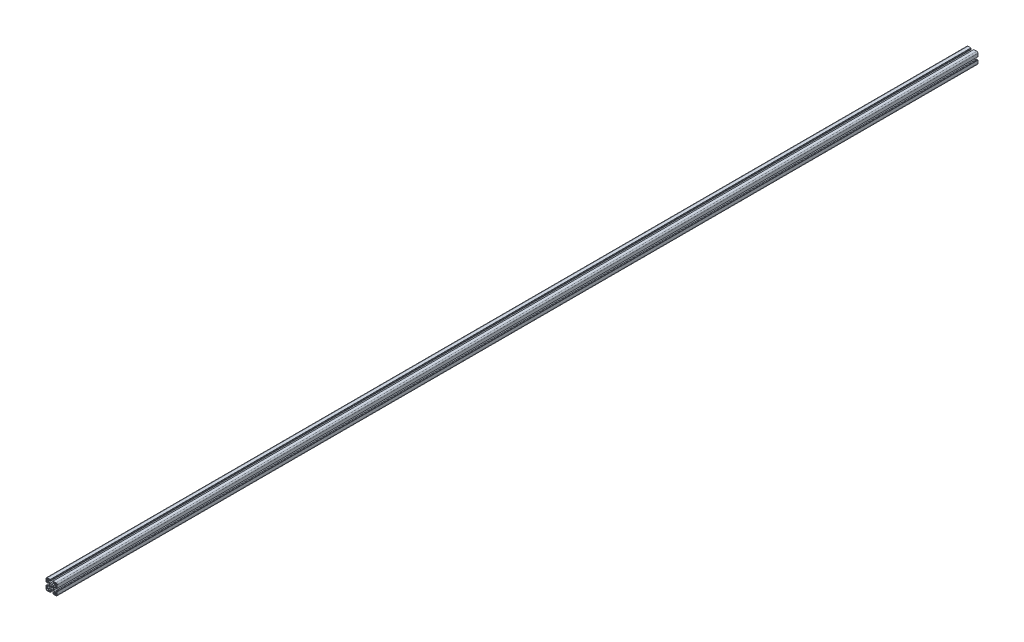
from build123d import *

# Parameters (mm, degrees)
EXTRUDE_1_DEPTH             = 3280
HOLE_WIZARD_2_D             = 6.6
HOLE_WIZARD_2_CBORE_D       = 11
HOLE_WIZARD_2_CBORE_DEPTH   = 6.8
HOLE_WIZARD_2_2_D           = 6.6
HOLE_WIZARD_2_2_CBORE_D     = 11
HOLE_WIZARD_2_2_CBORE_DEPTH = 6.8


with BuildPart() as part:
    # 草图1 → 凸台-拉伸1 (new body)
    with BuildSketch(Plane.XY):
        with BuildLine():
            Line((-18.9995, -4.100341675), (-18.9995, -5.100341675))
            Line((-18.9995, -5.100341675), (-19.9995, -5.100341675))
            Line((-19.9995, -5.100341675), (-19.9995, -15.500341675))
            ThreePointArc((-19.9995, -15.500341675), (-18.681480515, -18.682322191), (-15.4995, -20.000341675))
            Line((-15.4995, -20.000341675), (-5.0995, -20.000341675))
            Line((-5.0995, -20.000341675), (-5.0995, -19.000341675))
            Line((-5.0995, -19.000341675), (-4.0995, -19.000341675))
            Line((-4.0995, -19.000341675), (-4.0995, -15.500341675))
            Line((-4.0995, -15.500341675), (-6.5995, -15.500341675))
            Line((-6.5995, -15.500341675), (-6.5995, -16.500341675))
            ThreePointArc((-6.5995, -16.500341675), (-6.892393219, -17.207448457), (-7.5995, -17.500341675))
            Line((-7.5995, -17.500341675), (-9.7995, -17.500341675))
            ThreePointArc((-9.7995, -17.500341675), (-10.153053391, -17.353895066), (-10.2995, -17.000341675))
            Line((-10.2995, -17.000341675), (-10.2995, -11.997341675))
            Line((-10.2995, -11.997341675), (-5.9025, -7.600341675))
            Line((-5.9025, -7.600341675), (-0.5195, -7.600341675))
            Line((-0.5195, -7.600341675), (0.0005, -7.300341675))
            Line((0.0005, -7.300341675), (0.5195, -7.600341675))
            Line((0.5195, -7.600341675), (5.9035, -7.600341675))
            Line((5.9035, -7.600341675), (10.3005, -11.997341675))
            Line((10.3005, -11.997341675), (10.3005, -17.000341675))
            ThreePointArc((10.3005, -17.000341675), (10.154053391, -17.353895066), (9.8005, -17.500341675))
            Line((9.8005, -17.500341675), (7.6005, -17.500341675))
            ThreePointArc((7.6005, -17.500341675), (6.893393219, -17.207448457), (6.6005, -16.500341675))
            Line((6.6005, -16.500341675), (6.6005, -15.500341675))
            Line((6.6005, -15.500341675), (4.1005, -15.500341675))
            Line((4.1005, -15.500341675), (4.1005, -19.000341675))
            Line((4.1005, -19.000341675), (5.1005, -19.000341675))
            Line((5.1005, -19.000341675), (5.1005, -20.000341675))
            Line((5.1005, -20.000341675), (15.5005, -20.000341675))
            ThreePointArc((15.5005, -20.000341675), (18.682480515, -18.682322191), (20.0005, -15.500341675))
            Line((20.0005, -15.500341675), (20.0005, -5.100341675))
            Line((20.0005, -5.100341675), (19.0005, -5.100341675))
            Line((19.0005, -5.100341675), (19.0005, -4.100341675))
            Line((19.0005, -4.100341675), (15.5005, -4.100341675))
            Line((15.5005, -4.100341675), (15.5005, -6.600341675))
            Line((15.5005, -6.600341675), (16.5005, -6.600341675))
            ThreePointArc((16.5005, -6.600341675), (17.207606781, -6.893234894), (17.5005, -7.600341675))
            Line((17.5005, -7.600341675), (17.5005, -9.800341675))
            ThreePointArc((17.5005, -9.800341675), (17.354053391, -10.153895066), (17.0005, -10.300341675))
            Line((17.0005, -10.300341675), (11.9975, -10.300341675))
            Line((11.9975, -10.300341675), (7.6005, -5.903341675))
            Line((7.6005, -5.903341675), (7.6005, -0.520341675))
            Line((7.6005, -0.520341675), (7.3005, -0.000341675))
            Line((7.3005, -0.000341675), (7.6005, 0.519658325))
            Line((7.6005, 0.519658325), (7.6005, 5.902658325))
            Line((7.6005, 5.902658325), (11.9975, 10.299658325))
            Line((11.9975, 10.299658325), (17.0005, 10.299658325))
            ThreePointArc((17.0005, 10.299658325), (17.354053391, 10.153211715), (17.5005, 9.799658325))
            Line((17.5005, 9.799658325), (17.5005, 7.599658325))
            ThreePointArc((17.5005, 7.599658325), (17.207606781, 6.892551543), (16.5005, 6.599658325))
            Line((16.5005, 6.599658325), (15.5005, 6.599658325))
            Line((15.5005, 6.599658325), (15.5005, 4.099658325))
            Line((15.5005, 4.099658325), (19.0005, 4.099658325))
            Line((19.0005, 4.099658325), (19.0005, 5.099658325))
            Line((19.0005, 5.099658325), (20.0005, 5.099658325))
            Line((20.0005, 5.099658325), (20.0005, 15.499658325))
            ThreePointArc((20.0005, 15.499658325), (18.682480515, 18.68163884), (15.5005, 19.999658325))
            Line((15.5005, 19.999658325), (5.1005, 19.999658325))
            Line((5.1005, 19.999658325), (5.1005, 18.999658325))
            Line((5.1005, 18.999658325), (4.1005, 18.999658325))
            Line((4.1005, 18.999658325), (4.1005, 15.499658325))
            Line((4.1005, 15.499658325), (6.6005, 15.499658325))
            ThreePointArc((6.6005, 15.499658325), (6.393348977, 15.999658325), (6.6005, 16.499658325))
            ThreePointArc((6.6005, 16.499658325), (6.893393219, 17.206765106), (7.6005, 17.499658325))
            Line((7.6005, 17.499658325), (9.8005, 17.499658325))
            ThreePointArc((9.8005, 17.499658325), (10.154053391, 17.353211715), (10.3005, 16.999658325))
            Line((10.3005, 16.999658325), (10.3005, 11.996658325))
            Line((10.3005, 11.996658325), (5.9035, 7.599658325))
            Line((5.9035, 7.599658325), (0.5195, 7.599658325))
            Line((0.5195, 7.599658325), (0.0005, 7.299658325))
            Line((0.0005, 7.299658325), (-0.5195, 7.599658325))
            Line((-0.5195, 7.599658325), (-5.9025, 7.599658325))
            Line((-5.9025, 7.599658325), (-10.2995, 11.996658325))
            Line((-10.2995, 11.996658325), (-10.2995, 16.999658325))
            ThreePointArc((-10.2995, 16.999658325), (-10.153053391, 17.353211715), (-9.7995, 17.499658325))
            Line((-9.7995, 17.499658325), (-7.5995, 17.499658325))
            ThreePointArc((-7.5995, 17.499658325), (-6.892393219, 17.206765106), (-6.5995, 16.499658325))
            Line((-6.5995, 16.499658325), (-6.5995, 15.499658325))
            Line((-6.5995, 15.499658325), (-4.0995, 15.499658325))
            Line((-4.0995, 15.499658325), (-4.0995, 18.999658325))
            Line((-4.0995, 18.999658325), (-5.0995, 18.999658325))
            Line((-5.0995, 18.999658325), (-5.0995, 19.999658325))
            Line((-5.0995, 19.999658325), (-15.4995, 19.999658325))
            ThreePointArc((-15.4995, 19.999658325), (-18.681480515, 18.68163884), (-19.9995, 15.499658325))
            Line((-19.9995, 15.499658325), (-19.9995, 5.099658325))
            Line((-19.9995, 5.099658325), (-18.9995, 5.099658325))
            Line((-18.9995, 5.099658325), (-18.9995, 4.099658325))
            Line((-18.9995, 4.099658325), (-15.4995, 4.099658325))
            Line((-15.4995, 4.099658325), (-15.4995, 6.599658325))
            Line((-15.4995, 6.599658325), (-16.4995, 6.599658325))
            ThreePointArc((-16.4995, 6.599658325), (-17.206606781, 6.892551543), (-17.4995, 7.599658325))
            Line((-17.4995, 7.599658325), (-17.4995, 9.799658325))
            ThreePointArc((-17.4995, 9.799658325), (-17.353053391, 10.153211715), (-16.9995, 10.299658325))
            Line((-16.9995, 10.299658325), (-11.9965, 10.299658325))
            Line((-11.9965, 10.299658325), (-7.5995, 5.902658325))
            Line((-7.5995, 5.902658325), (-7.5995, 0.519658325))
            Line((-7.5995, 0.519658325), (-7.2995, -0.000341675))
            Line((-7.2995, -0.000341675), (-7.5995, -0.520341675))
            Line((-7.5995, -0.520341675), (-7.5995, -5.903341675))
            Line((-7.5995, -5.903341675), (-11.9965, -10.300341675))
            Line((-11.9965, -10.300341675), (-16.9995, -10.300341675))
            ThreePointArc((-16.9995, -10.300341675), (-17.353053391, -10.153895066), (-17.4995, -9.800341675))
            Line((-17.4995, -9.800341675), (-17.4995, -7.600341675))
            ThreePointArc((-17.4995, -7.600341675), (-17.206606781, -6.893234894), (-16.4995, -6.600341675))
            Line((-16.4995, -6.600341675), (-15.4995, -6.600341675))
            Line((-15.4995, -6.600341675), (-15.4995, -4.100341675))
            Line((-15.4995, -4.100341675), (-18.9995, -4.100341675))
        make_face()
        with BuildLine():
            Line((15.5005, -18.000341675), (11.8005, -18.000341675))
            Line((11.8005, -18.000341675), (11.8005, -11.800341675))
            Line((11.8005, -11.800341675), (18.0005, -11.800341675))
            Line((18.0005, -11.800341675), (18.0005, -15.500341675))
            ThreePointArc((18.0005, -15.500341675), (17.268266953, -17.268108628), (15.5005, -18.000341675))
        make_face(mode=Mode.SUBTRACT)
        with BuildLine():
            Line((18.0005, 11.799658325), (11.8005, 11.799658325))
            Line((11.8005, 11.799658325), (11.8005, 17.999658325))
            Line((11.8005, 17.999658325), (15.5005, 17.999658325))
            ThreePointArc((15.5005, 17.999658325), (17.268266953, 17.267425278), (18.0005, 15.499658325))
            Line((18.0005, 15.499658325), (18.0005, 11.799658325))
        make_face(mode=Mode.SUBTRACT)
        with BuildLine():
            Line((-1.8145, -2.875341675), (-3.004391671, -4.066450004))
            Line((-3.004391671, -4.066450004), (-4.065608329, -3.005233346))
            Line((-4.065608329, -3.005233346), (-2.8745, -1.815341675))
            ThreePointArc((-2.8745, -1.815341675), (-3.399473913, -0.000341675), (-2.8745, 1.814658325))
            Line((-2.8745, 1.814658325), (-4.064391671, 3.005766654))
            Line((-4.064391671, 3.005766654), (-3.004391671, 4.065766654))
            Line((-3.004391671, 4.065766654), (-1.8145, 2.874658325))
            ThreePointArc((-1.8145, 2.874658325), (0, 3.399316649), (1.8145, 2.874658325))
            Line((1.8145, 2.874658325), (3.0055, 4.065658325))
            Line((3.0055, 4.065658325), (4.066608329, 3.004549996))
            Line((4.066608329, 3.004549996), (2.8755, 1.814658325))
            ThreePointArc((2.8755, 1.814658325), (3.400473913, -0.000341675), (2.8755, -1.815341675))
            Line((2.8755, -1.815341675), (4.066608329, -3.005233346))
            Line((4.066608329, -3.005233346), (3.0055, -4.066341675))
            Line((3.0055, -4.066341675), (1.8145, -2.875341675))
            ThreePointArc((1.8145, -2.875341675), (0, -3.4), (-1.8145, -2.875341675))
        make_face(mode=Mode.SUBTRACT)
        with BuildLine():
            Line((-17.9995, -15.500341675), (-17.9995, -11.800341675))
            Line((-17.9995, -11.800341675), (-11.7995, -11.800341675))
            Line((-11.7995, -11.800341675), (-11.7995, -18.000341675))
            Line((-11.7995, -18.000341675), (-15.4995, -18.000341675))
            ThreePointArc((-15.4995, -18.000341675), (-17.267266953, -17.268108628), (-17.9995, -15.500341675))
        make_face(mode=Mode.SUBTRACT)
        with BuildLine():
            Line((-11.7995, 17.999658325), (-11.7995, 11.799658325))
            Line((-11.7995, 11.799658325), (-17.9995, 11.799658325))
            Line((-17.9995, 11.799658325), (-17.9995, 15.499658325))
            ThreePointArc((-17.9995, 15.499658325), (-17.267266953, 17.267425278), (-15.4995, 17.999658325))
            Line((-15.4995, 17.999658325), (-11.7995, 17.999658325))
        make_face(mode=Mode.SUBTRACT)
    extrude(amount=-EXTRUDE_1_DEPTH)

    # Hole Wizard 2 (through all)
    with Locations(Plane(origin=(0.000841675, -20.000341675, 0), x_dir=(0, 0, 1), z_dir=(0, -1, 0))):
        with Locations((-80, 0.000341675), (-1080, 0.000341675), (-2200, 0.000341675), (-3200, 0.000341675)):
            CounterBoreHole(HOLE_WIZARD_2_D / 2, HOLE_WIZARD_2_CBORE_D / 2, HOLE_WIZARD_2_CBORE_DEPTH)

    # Hole Wizard 2 2 (through all)
    with Locations(Plane(origin=(0, 19.999658325, 0), x_dir=(1, 0, 0), z_dir=(0, 1, 0))):
        with Locations((0.0005, 1080), (0.0005, 1640), (0.0005, 2200), (0.0005, 3200), (0.0005, 80)):
            CounterBoreHole(HOLE_WIZARD_2_2_D / 2, HOLE_WIZARD_2_2_CBORE_D / 2, HOLE_WIZARD_2_2_CBORE_DEPTH)


solid = part.part
